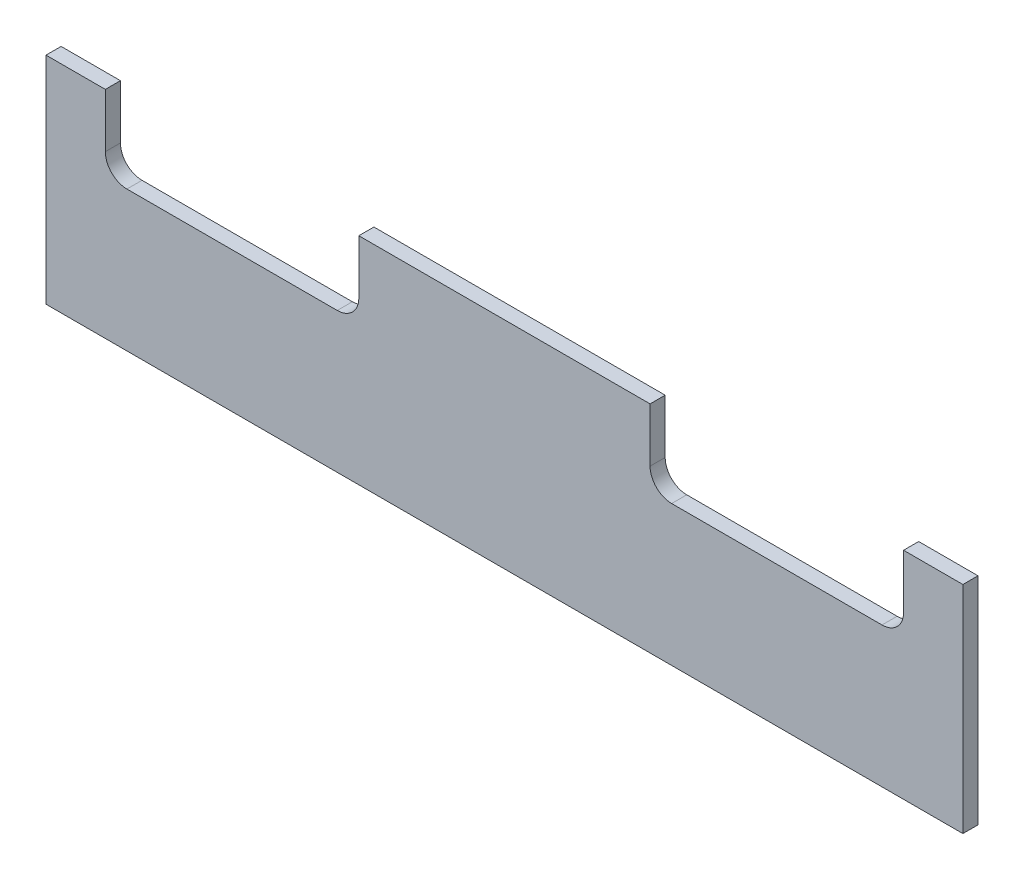
from build123d import *

# Parameters (mm, degrees)
SKETCH_1_W          = 850
SKETCH_1_H          = 200
EXTRUDE_1_DEPTH     = 14
CUT_EXTRUDE_1_REACH = 438.831
SKETCH_2_W          = 235
SKETCH_2_H          = 70
FILLET_1_R          = 20


with BuildPart() as part:
    # 草图1 → 凸台-拉伸1 (new body)
    with BuildSketch(Plane.XY):
        Rectangle(SKETCH_1_W, SKETCH_1_H)
    extrude(amount=EXTRUDE_1_DEPTH)

    # 草图2 → 切除-拉伸1 (cut, up to next)
    with BuildSketch(Plane(origin=(0, 0, 0), x_dir=(-1, 0, 0), z_dir=(0, 0, -1)), mode=Mode.PRIVATE) as cut_extrude_1_sk1:
        with Locations((252.5, 65)):
            Rectangle(SKETCH_2_W, SKETCH_2_H)
    cut_extrude_1_tool1 = extrude(cut_extrude_1_sk1.sketch, amount=-CUT_EXTRUDE_1_REACH, mode=Mode.PRIVATE) & part.part
    # 草图2 → 切除-拉伸1 (cut, up to next)
    with BuildSketch(Plane(origin=(0, 0, 0), x_dir=(-1, 0, 0), z_dir=(0, 0, -1)), mode=Mode.PRIVATE) as cut_extrude_1_sk2:
        with Locations((-252.5, 65)):
            Rectangle(SKETCH_2_W, SKETCH_2_H)
    cut_extrude_1_tool2 = extrude(cut_extrude_1_sk2.sketch, amount=-CUT_EXTRUDE_1_REACH, mode=Mode.PRIVATE) & part.part
    add(cut_extrude_1_tool1.solids().sort_by_distance((-252.5, 65, 0))[0], mode=Mode.SUBTRACT)
    add(cut_extrude_1_tool2.solids().sort_by_distance((252.5, 65, 0))[0], mode=Mode.SUBTRACT)

    # 圆角1
    fillet_1_edges = [part.edges().sort_by_distance(p)[0] for p in [
        (-370, 30, 7),
        (-135, 30, 7),
        (135, 30, 7),
        (370, 30, 7),
    ]]
    fillet(fillet_1_edges, radius=FILLET_1_R)


solid = part.part
